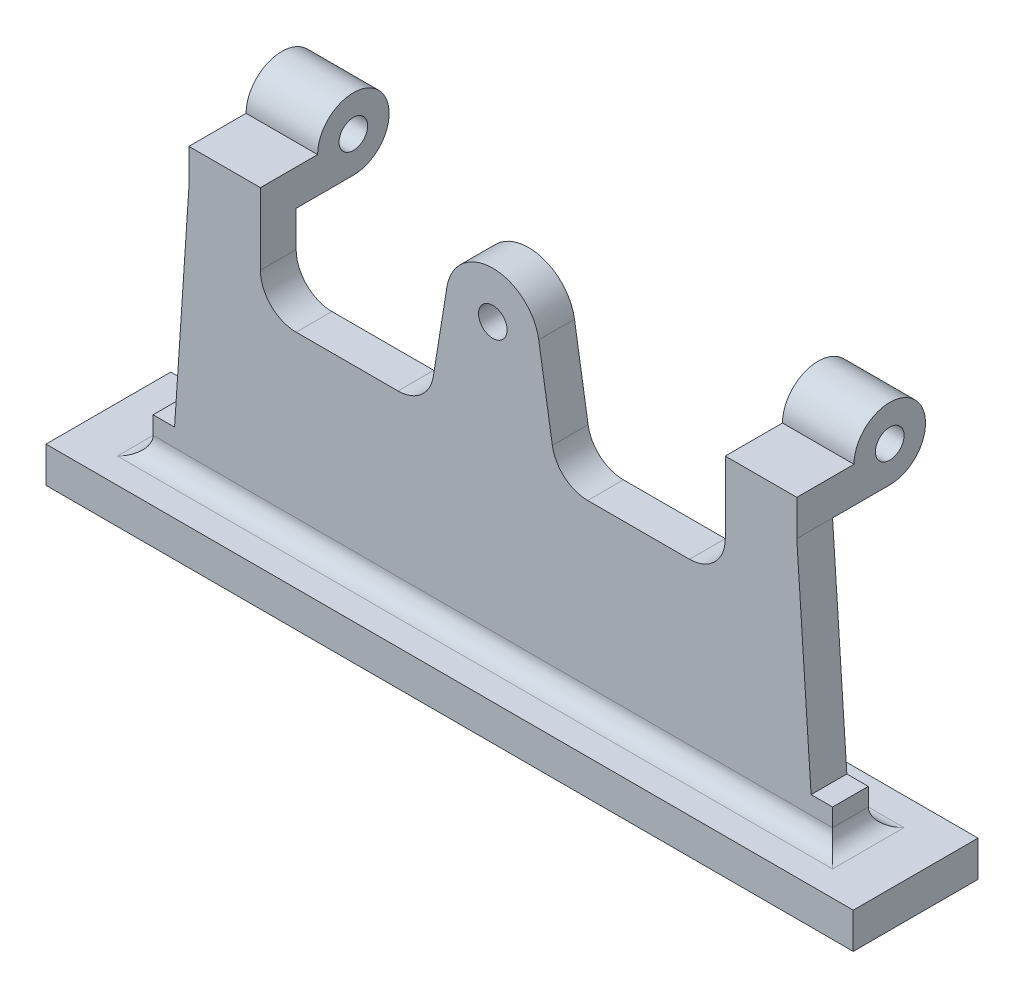
from build123d import *

# Parameters (mm, degrees)
SKETCH1_R           = 4
BOSS_EXTRUDE1_DEPTH = 10
SKETCH2_W           = 225.743396996
SKETCH2_H           = 34.886278096
BOSS_EXTRUDE2_DEPTH = 10
SKETCH3_R           = 4
BOSS_EXTRUDE3_DEPTH = 20
FILLET1_R           = 5


with BuildPart() as part:
    # Sketch1 → Boss-Extrude1 (new body)
    with BuildSketch(Plane.XY):
        with BuildLine():
            Line((-85, -10), (-89, -70))
            Line((-89, -70), (-95, -70))
            Line((-95, -70), (-95, -80))
            Line((-95, -80), (95, -80))
            Line((95, -80), (95, -70))
            Line((95, -70), (89, -70))
            Line((89, -70), (85, -10))
            Line((85, -10), (65, -10))
            Line((65, -10), (65, -20))
            ThreePointArc((65, -20), (62.071067812, -27.071067812), (55, -30))
            Line((55, -30), (26.518096199, -30))
            ThreePointArc((26.518096199, -30), (20.033617948, -27.612591006), (16.645360037, -21.590308363))
            Line((16.645360037, -21.590308363), (12.83455701, 2.067400872))
            ThreePointArc((12.83455701, 2.067400872), (0, 13), (-12.83455701, 2.067400872))
            Line((-12.83455701, 2.067400872), (-16.645360037, -21.590308363))
            ThreePointArc((-16.645360037, -21.590308363), (-20.033617948, -27.612591006), (-26.518096199, -30))
            Line((-26.518096199, -30), (-55, -30))
            ThreePointArc((-55, -30), (-62.071067812, -27.071067812), (-65, -20))
            Line((-65, -20), (-65, -10))
            Line((-65, -10), (-85, -10))
        make_face()
        Circle(SKETCH1_R, mode=Mode.SUBTRACT)
    extrude(amount=BOSS_EXTRUDE1_DEPTH)

    # Sketch2 → Boss-Extrude2 (add)
    with BuildSketch(Plane(origin=(0, -80, 0), x_dir=(-1, 0, 0), z_dir=(0, -1, 0))):
        with Locations((0, -4.638757859)):
            Rectangle(SKETCH2_W, SKETCH2_H)
    extrude(amount=BOSS_EXTRUDE2_DEPTH)

    # Sketch3 → Boss-Extrude3 (add)
    with BuildSketch(Plane(origin=(-65, 0, 0), x_dir=(0, 0, -1), z_dir=(1, 0, 0))):
        with BuildLine():
            Line((6, 0), (-10, 0))
            Line((-10, 0), (-10, -10))
            Line((-10, -10), (16, -10))
            ThreePointArc((16, -10), (23.071067812, 7.071067812), (6, 0))
        make_face()
        with Locations(Location((16, 0, 0), (0, 0, 90))):
            Circle(SKETCH3_R, mode=Mode.SUBTRACT)
    boss_extrude3 = extrude(amount=-BOSS_EXTRUDE3_DEPTH)

    # Mirror1: Boss-Extrude3 across plane
    add(boss_extrude3.mirror(Plane(origin=(0, 0, 0), x_dir=(0, 0, 1), z_dir=(1, 0, 0))))

    # Fillet1
    fillet1_edges = [part.edges().sort_by_distance(p)[0] for p in [
        (0, -80, 0),
        (95, -80, 5),
        (-95, -80, 5),
        (0, -80, 10),
    ]]
    fillet(fillet1_edges, radius=FILLET1_R)


solid = part.part
